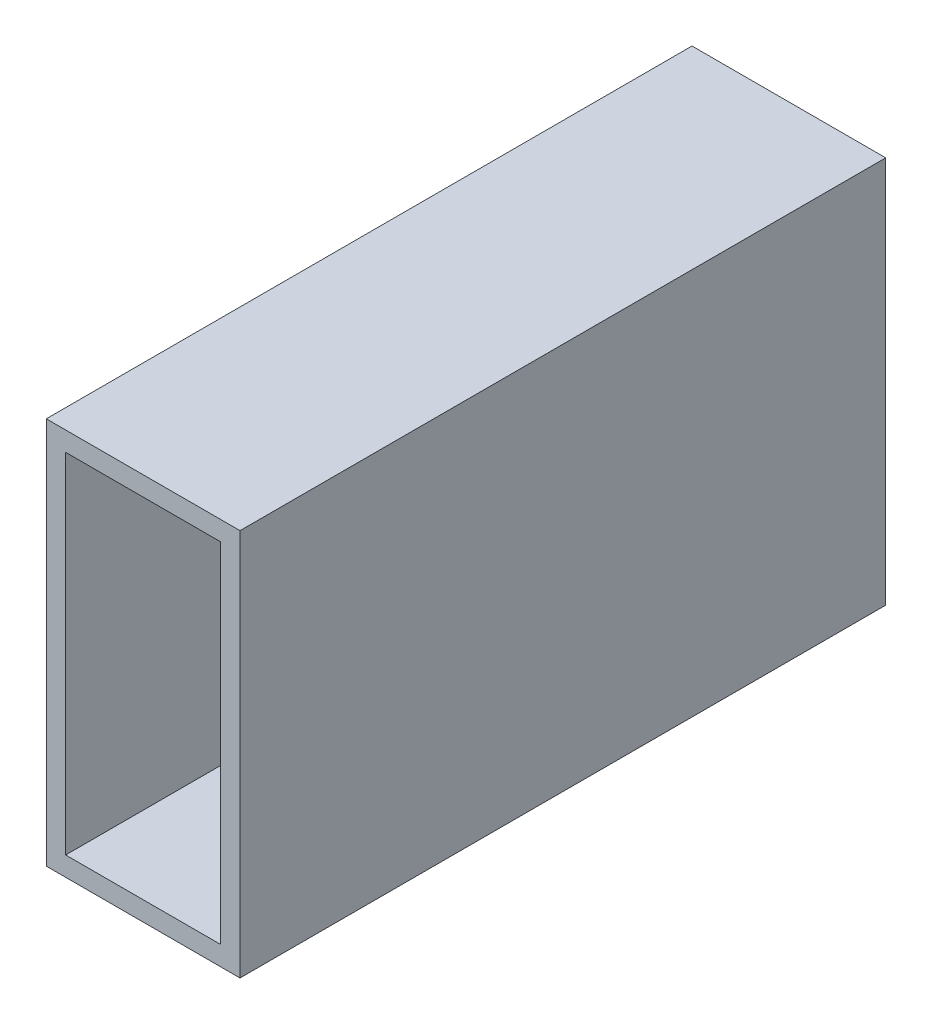
SolidWorks part; units mm, degrees
material "Q235A"
ref_plane "前视基准面" through (0, 0, 0) normal (0, 0, 1) x (1, 0, 0)
ref_plane "上视基准面" through (0, 0, 0) normal (0, 1, 0) x (1, 0, 0)
ref_plane "右视基准面" through (0, 0, 0) normal (1, 0, 0) x (0, 0, -1)
sketch "草图1" plane through (0, 0, 0) normal (0, 0, 1) x (1, 0, 0)
  line L1 (-15, -30) -> (15, -30)
  line L2 (-15, -30) -> (-15, 30)
  line L3 (-15, 30) -> (15, 30)
  line L4 (15, -30) -> (15, 30)
  line L5 (-15, -30) -> (15, 30) construction
  line L6 (-15, 30) -> (15, -30) construction
  point P0 (0, 0)
  dimension "D1" = 30
  dimension "D2" = 60
extrude "拉伸-薄壁1" add sketch "草图1" along normal blind 100 thin thin type one direction reverse wall 3
